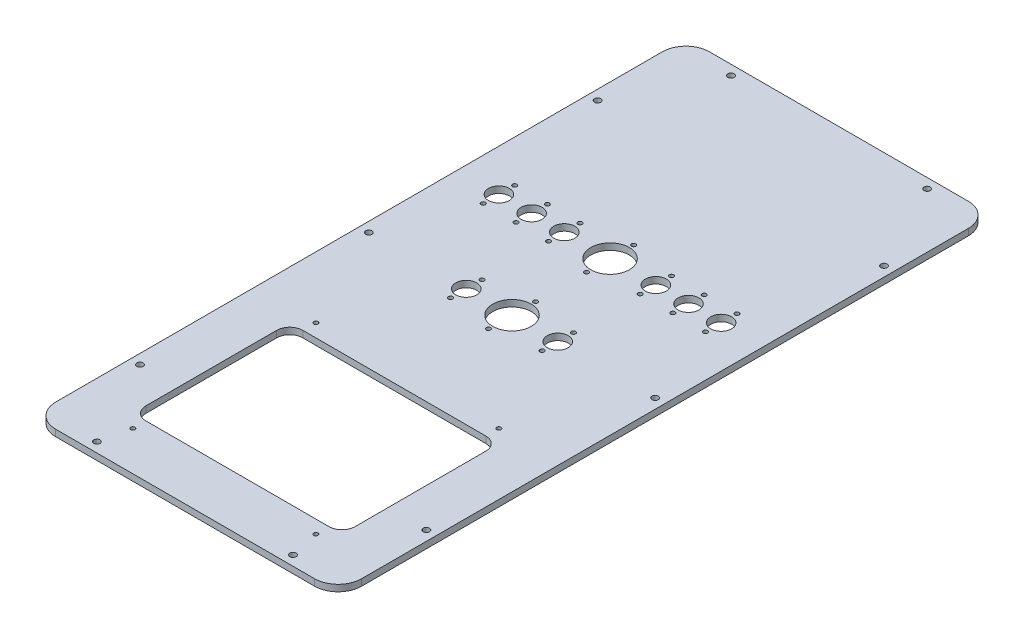
from build123d import *

# Parameters (mm, degrees)
SKETCH1_W            = 234
SKETCH1_H            = 500
BOSS_EXTRUDE1_DEPTH  = 2.5
M4_CLEARANCE_HOLE1_D = 4.8
FILLET1_R            = 18
M4_TAPPED_HOLE7_D    = 3.3
SKETCH4_R            = 14.75
SKETCH4_R_2          = 8
CUT_EXTRUDE6_DEPTH   = 277.068831997
M4_TAPPED_HOLE3_D    = 3.3
SKETCH9_R            = 14.75
CUT_EXTRUDE3_DEPTH   = 277.068831997
M4_TAPPED_HOLE4_D    = 3.3
SKETCH12_W           = 160
SKETCH12_H           = 120
CUT_EXTRUDE4_DEPTH   = 277.068831997
FILLET2_R            = 10


with BuildPart() as part:
    # Sketch1 → Boss-Extrude1 (new, symmetric)
    with BuildSketch(Plane(origin=(0, 0, 0), x_dir=(1, 0, 0), z_dir=(0, 1, 0))):
        Rectangle(SKETCH1_W, SKETCH1_H)
    extrude(amount=BOSS_EXTRUDE1_DEPTH, both=True)

    # M4 Clearance Hole1 (through all)
    with Locations(Plane(origin=(-75, 2.5, -242.5), x_dir=(0, 0, 1), z_dir=(0, 1, 0))):
        with Locations((0, 0), (0, 150), (67.5, 184.5), (67.5, -34.5), (242.5, 184.5), (242.5, -34.5), (417.5, -34.5), (417.5, 184.5), (485, 0), (485, 150)):
            Hole(M4_CLEARANCE_HOLE1_D / 2)

    # Fillet1
    fillet1_edges = [part.edges().sort_by_distance(p)[0] for p in [
        (117, 0, 250),
        (-117, 0, 250),
        (-117, 0, -250),
        (117, 0, -250),
    ]]
    fillet(fillet1_edges, radius=FILLET1_R)

    # M4 Tapped Hole7 (through all)
    with Locations(Plane(origin=(-85, 2.5, -87), x_dir=(0, 0, 1), z_dir=(0, 1, 0))):
        with Locations((0, 0), (24, 0), (24, 25), (0, 25), (0, 50), (24, 50), (-6, 85), (30, 85), (0, 120), (24, 120), (0, 145), (24, 145), (0, 170), (24, 170), (75, 120), (99, 120), (75, 50), (99, 50)):
            Hole(M4_TAPPED_HOLE7_D / 2)

    # Sketch4 → Cut-Extrude6 (cut, through all)
    with BuildSketch(Plane(origin=(0, 2.5, 0), x_dir=(1, 0, 0), z_dir=(0, 1, 0))):
        with Locations(Location((0, 75, 0), (0, 0, 270))):
            Circle(SKETCH4_R)
        with Locations(Location((-35, 75, 0), (0, 0, 270))):
            Circle(SKETCH4_R_2)
        with Locations(Location((35, 75, 0), (0, 0, 270))):
            Circle(SKETCH4_R_2)
        with Locations(Location((-60, 75, 0), (0, 0, 270))):
            Circle(SKETCH4_R_2)
        with Locations(Location((-85, 75, 0), (0, 0, 270))):
            Circle(SKETCH4_R_2)
        with Locations(Location((60, 75, 0), (0, 0, 270))):
            Circle(SKETCH4_R_2)
        with Locations(Location((85, 75, 0), (0, 0, 270))):
            Circle(SKETCH4_R_2)
        with Locations(Location((35, 0, 0), (0, 0, 270))):
            Circle(SKETCH4_R_2)
        with Locations(Location((-35, 0, 0), (0, 0, 270))):
            Circle(SKETCH4_R_2)
    extrude(amount=-CUT_EXTRUDE6_DEPTH, mode=Mode.SUBTRACT)

    # M4 Tapped Hole3 (through all)
    with Locations(Plane(origin=(0, 2.5, -18), x_dir=(0, 0, 1), z_dir=(0, 1, 0))):
        with Locations((0, 0), (36, 0)):
            Hole(M4_TAPPED_HOLE3_D / 2)

    # Sketch9 → Cut-Extrude3 (cut, through all)
    with BuildSketch(Plane(origin=(0, 2.5, 0), x_dir=(1, 0, 0), z_dir=(0, 1, 0))):
        with Locations(Location((0, 0, 0), (0, 0, 270))):
            Circle(SKETCH9_R)
    extrude(amount=-CUT_EXTRUDE3_DEPTH, mode=Mode.SUBTRACT)

    # M4 Tapped Hole4 (through all)
    with Locations(Plane(origin=(-70, 2.5, 80), x_dir=(0, 0, 1), z_dir=(0, 1, 0))):
        with Locations((0, 0), (0, 140), (140, 140), (140, 0)):
            Hole(M4_TAPPED_HOLE4_D / 2)

    # Sketch12 → Cut-Extrude4 (cut, through all)
    with BuildSketch(Plane(origin=(0, 2.5, 0), x_dir=(1, 0, 0), z_dir=(0, 1, 0))):
        with Locations((0, -150)):
            Rectangle(SKETCH12_W, SKETCH12_H)
    extrude(amount=-CUT_EXTRUDE4_DEPTH, mode=Mode.SUBTRACT)

    # Fillet2
    fillet2_edges = [part.edges().sort_by_distance(p)[0] for p in [
        (80, 0, 90),
        (80, 0, 210),
        (-80, 0, 210),
        (-80, 0, 90),
    ]]
    fillet(fillet2_edges, radius=FILLET2_R)


solid = part.part
